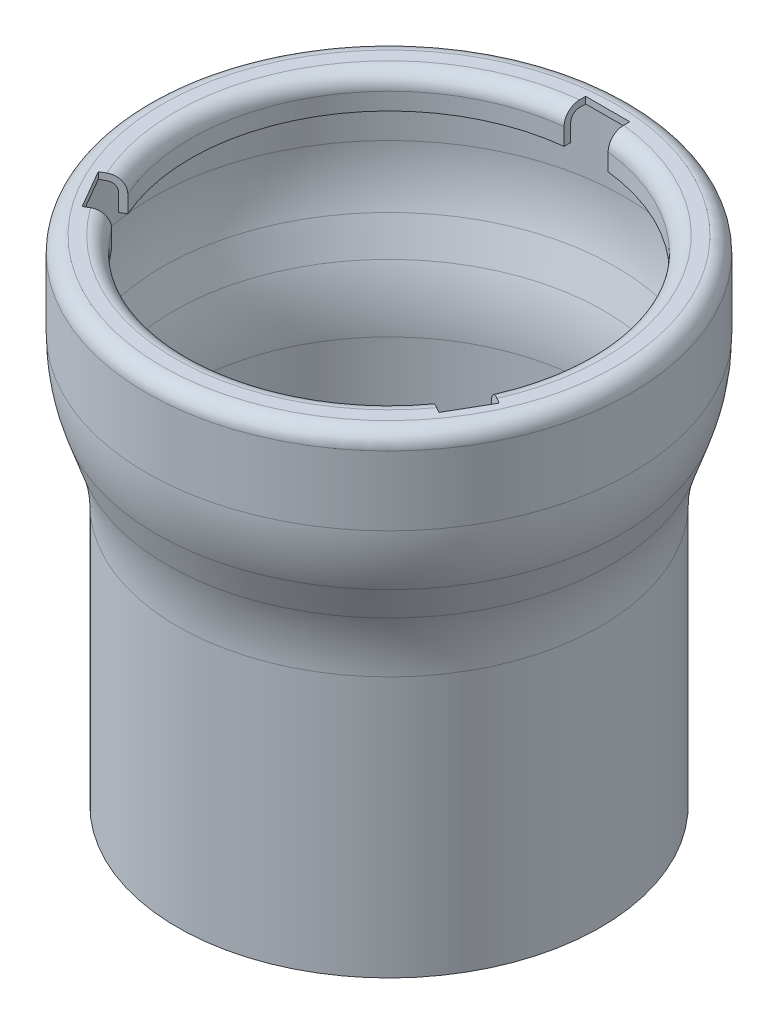
from build123d import *

# Parameters (mm, degrees)
SKETCH2_W          = 10
SKETCH2_H          = 19.823502967
CUT_EXTRUDE1_DEPTH = 10
CIRPATTERN1_COUNT  = 3


with BuildPart() as part:
    # Sketch1 → Revolve1 (revolve)
    with BuildSketch(Plane.XY, mode=Mode.PRIVATE) as revolve1_sk:
        with BuildLine():
            Line((48, 0), (48, 59.156721496))
            ThreePointArc((48, 59.156721496), (48.557497865, 65.81172152), (50.214451266, 72.281214129))
            Line((50.214451266, 72.281214129), (52.785548734, 79.683430077))
            ThreePointArc((52.785548734, 79.683430077), (54.442502135, 86.152922686), (55, 92.80792271))
            Line((55, 92.80792271), (55, 108.5))
            ThreePointArc((55, 108.5), (53.974873734, 110.974873734), (51.5, 112))
            Line((51.5, 112), (48.5, 112))
            ThreePointArc((48.5, 112), (46.025126266, 110.974873734), (45, 108.5))
            Line((45, 108.5), (45, 104.615384615))
            Line((45, 104.615384615), (46.5, 104.615384615))
            Line((46.5, 104.615384615), (46.5, 108.5))
            ThreePointArc((46.5, 108.5), (47.085786438, 109.914213562), (48.5, 110.5))
            Line((48.5, 110.5), (51.5, 110.5))
            ThreePointArc((51.5, 110.5), (52.914213562, 109.914213562), (53.5, 108.5))
            Line((53.5, 108.5), (53.5, 92.80792271))
            ThreePointArc((53.5, 92.80792271), (52.963408305, 86.402485187), (51.368590657, 80.175598551))
            Line((51.368590657, 80.175598551), (48.797493188, 72.773382602))
            ThreePointArc((48.797493188, 72.773382602), (47.078404035, 66.061284021), (46.5, 59.156721496))
            Line((46.5, 59.156721496), (46.5, 0))
            Line((46.5, 0), (48, 0))
        make_face()
    revolve(revolve1_sk.sketch.rotate(Axis((0, 0, 0), (0, 1, 0)), 90), axis=Axis((0, 0, 0), (0, 1, 0)))

    # Sketch2 → Cut-Extrude1 (cut)
    with BuildSketch(Plane(origin=(0, 112, 0), x_dir=(1, 0, 0), z_dir=(0, 1, 0))):
        with Locations((0, 39.713792094)):
            Rectangle(SKETCH2_W, SKETCH2_H)
    cut_extrude1 = extrude(amount=-CUT_EXTRUDE1_DEPTH, mode=Mode.SUBTRACT)

    # CirPattern1: Cut-Extrude1 ×3 about axis
    cirpattern1_axis = Axis((0, 0, 0), (0, 1, 0))
    for i in range(1, CIRPATTERN1_COUNT):
        add(cut_extrude1.rotate(cirpattern1_axis, i * 360 / CIRPATTERN1_COUNT), mode=Mode.SUBTRACT)


solid = part.part
